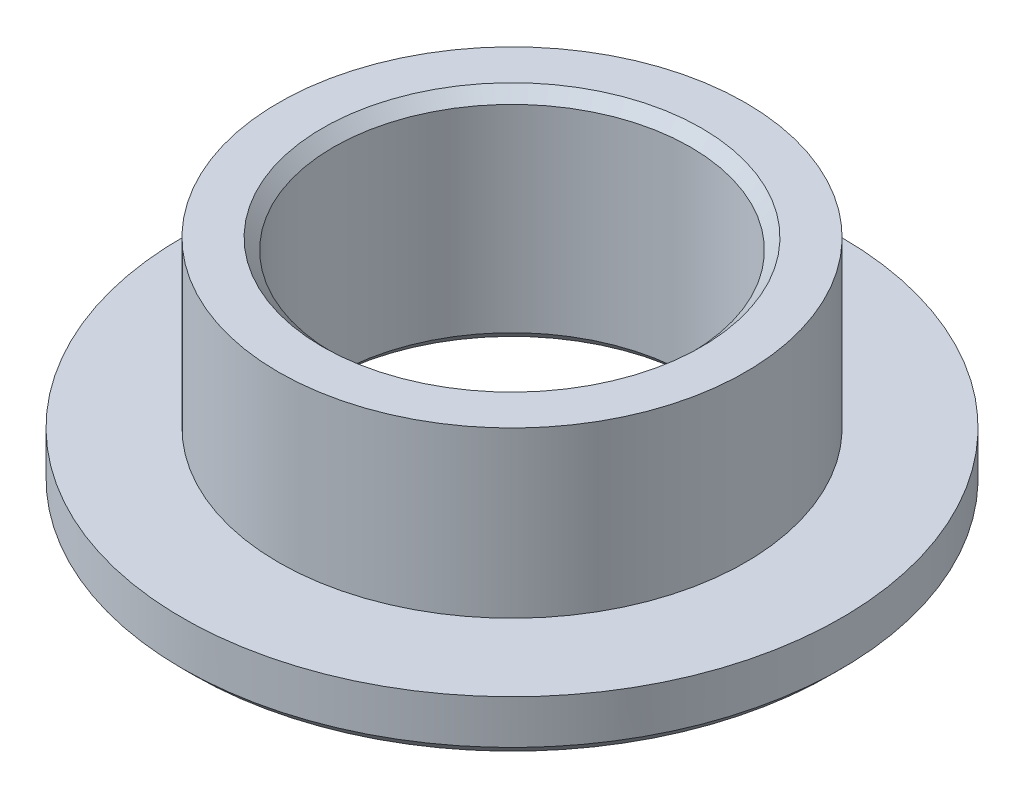
SolidWorks part; units mm, degrees
ref_plane "Front Plane" through (0, 0, 0) normal (0, 0, 1) x (1, 0, 0)
ref_plane "Top Plane" through (0, 0, 0) normal (0, 1, 0) x (1, 0, 0)
ref_plane "Right Plane" through (0, 0, 0) normal (1, 0, 0) x (0, 0, -1)
sketch "Sketch1" plane through (0, 0, 0) normal (0, 0, 1) x (1, 0, 0)
  line L0 (-32.5, 0) -> (-32.5, 40)
  line L1 (-32.5, 40) -> (-42.5, 40)
  line L2 (-42.5, 40) -> (-42.5, 10)
  line L3 (-42.5, 10) -> (-60, 10)
  line L4 (-60, 10) -> (-60, 0)
  line L5 (-60, 0) -> (-32.5, 0)
  line L6 (0, 0) -> (0, 57.3198) construction
  dimension "D1" = 32.5
  dimension "D2" = 42.5
  dimension "D3" = 60
  dimension "D4" = 40
  dimension "D5" = 30
  dimension "D6" = 40
revolve "Revolve1" add sketch "Sketch1" angle 360 about L6
chamfer "Chamfer1" distance 2 angle 45 3 edges at (0, 40, -32.5) (0, 0, -32.5) (0, 0, -60)
